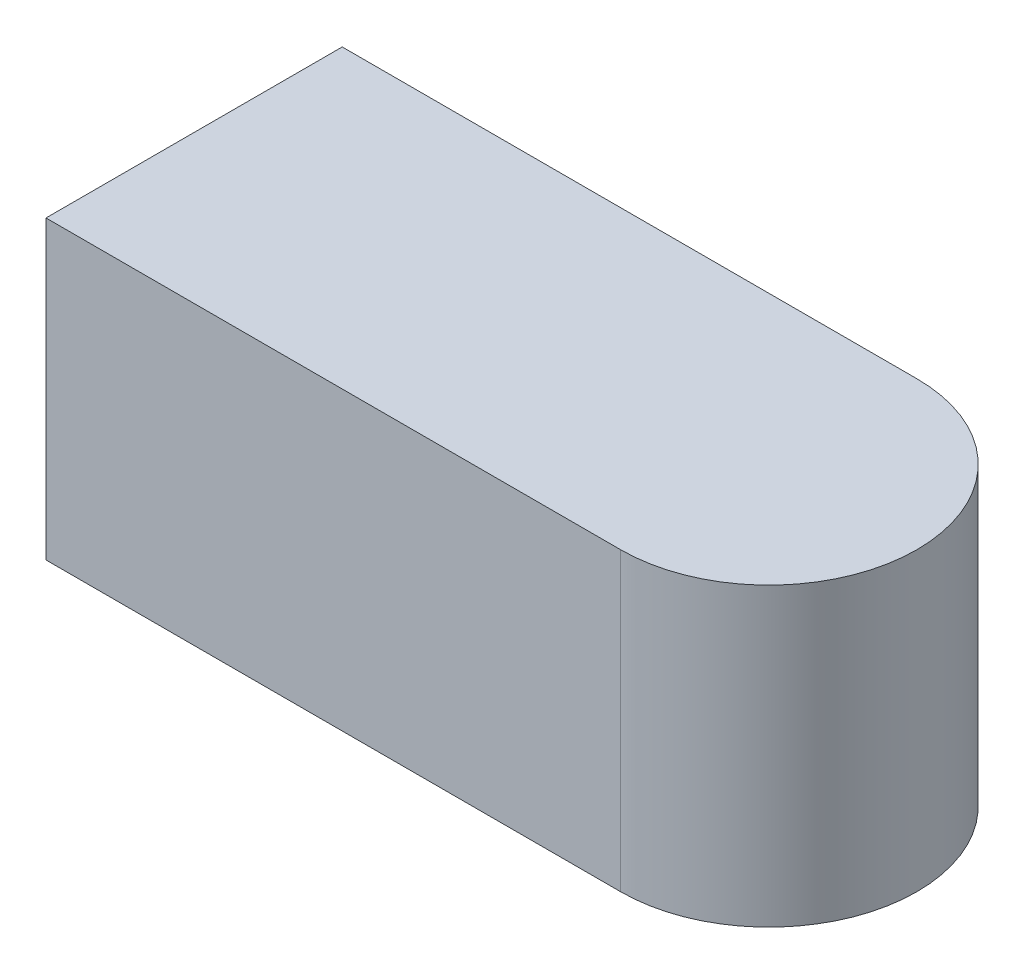
SolidWorks part; units mm, degrees
material "AISI 4340 Steel, normalized"
ref_plane "Front" through (0, 0, 0) normal (0, 0, 1) x (1, 0, 0)
ref_plane "Top" through (0, 0, 0) normal (0, 1, 0) x (1, 0, 0)
ref_plane "Right" through (0, 0, 0) normal (1, 0, 0) x (0, 0, -1)
sketch "Sketch1" plane through (0, 0, 0) normal (0, 1, 0) x (1, 0, 0)
  line L1 (0, 3.175) -> (12.319, 3.175)
  line L2 (0, 3.175) -> (0, -3.175)
  line L3 (0, -3.175) -> (12.319, -3.175)
  arc A0 (12.319, -3.175) -> (12.319, 3.175) centre (12.319, 0) ccw
  point P7 (0, 0)
  dimension "D3" = 6.35
  dimension "D1" = 6.35
  dimension "D2" = 12.319
extrude "Boss-Extrude1" add sketch "Sketch1" along normal mid plane 6.35
sketch "Sketch2" plane through (0, 0, 0) normal (-1, 0, 0) x (0, 0, 1)
  circle A0 centre (0, 0) radius 2.4384
  dimension "D1" = 4.8768
extrude "Cut-Extrude1" cut sketch "Sketch2" against normal blind 11.1125
sketch "Sketch3" plane through (0, 0, 0) normal (0, 1, 0) x (1, 0, 0)
  line L0 (0, 0) -> (13.9176, 0) construction
  line L1 (13.9176, 0) -> (11.1125, -2.4384)
  line L2 (11.1125, -2.4384) -> (0, -2.4384)
  line L3 (0, -2.4384) -> (0, 0)
  line L4 (0, 0) -> (13.9176, 0)
  dimension "D1" = 41
  dimension "D2" = 11.1125
revolve "Cut-Revolve1" cut sketch "Sketch3" angle 360 about L0
